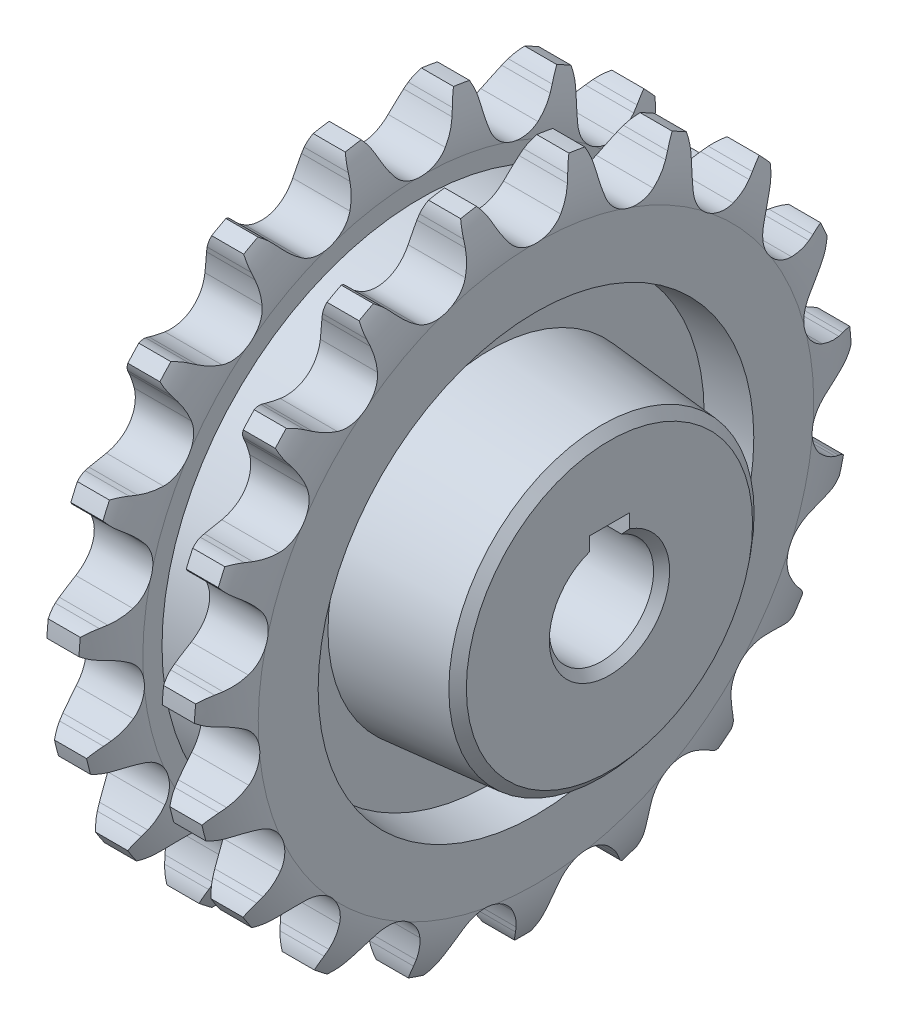
from build123d import *
from OCP.BRepFilletAPI import BRepFilletAPI_MakeChamfer

# Parameters (mm, degrees)
CUT_EXTRUDE1_DEPTH = 5.475375
CIRPATTERN1_COUNT  = 19
LPATTERN1_COUNT    = 2
LPATTERN1_PITCH    = 14.38
CHAMFER1_SIZE      = 1
CHAMFER1_SIZE2     = 1.100062868
SKETCH4_W          = 5
SKETCH4_H          = 2.799999952
CUT_EXTRUDE4_DEPTH = 71.401283385


with BuildPart() as part:
    # Sketch1 → Revolve1 (revolve)
    with BuildSketch(Plane.XY, mode=Mode.PRIVATE) as revolve1_sk:
        with BuildLine():
            Line((-3.65025, 27.149639763), (-3.65025, 34.619639763))
            ThreePointArc((-3.65025, 34.619639763), (-3.245836945, 37.918781526), (-1.99925, 41))
            Line((-1.99925, 41), (1.99925, 41))
            ThreePointArc((1.99925, 41), (3.245836945, 37.918781526), (3.65025, 34.619639763))
            Line((3.65025, 34.619639763), (3.65025, 27.149639763))
            Line((3.65025, 27.149639763), (-3.65025, 27.149639763))
        make_face()
    revolve(revolve1_sk.sketch.rotate(Axis((-6.35, 0, 0), (1, 0, 0)), 90), axis=Axis((-6.35, 0, 0), (1, 0, 0)))

    # Sketch2 → Cut-Extrude1 (cut, symmetric)
    with BuildSketch(Plane(origin=(0, 0, 0), x_dir=(0, 0, -1), z_dir=(1, 0, 0))):
        with BuildLine():
            Line((4.552244709, 38.426451297), (4.858741585, 39.1448403))
            ThreePointArc((4.858741585, 39.1448403), (5.250930322, 39.90290393), (5.750855114, 40.594675334))
            ThreePointArc((5.750855114, 40.594675334), (0, 41), (-5.750855114, 40.594675334))
            ThreePointArc((-5.750855114, 40.594675334), (-5.250930322, 39.90290393), (-4.858741585, 39.1448403))
            Line((-4.858741585, 39.1448403), (-4.552244709, 38.426451297))
            ThreePointArc((-4.552244709, 38.426451297), (-3.937302758, 37.212676935), (-3.168676608, 36.089905522))
            ThreePointArc((-3.168676608, 36.089905522), (0, 34.549839763), (3.168676608, 36.089905522))
            ThreePointArc((3.168676608, 36.089905522), (3.937302758, 37.212676935), (4.552244709, 38.426451297))
        make_face()
    cut_extrude1 = extrude(amount=CUT_EXTRUDE1_DEPTH, both=True, mode=Mode.SUBTRACT)

    # CirPattern1: Cut-Extrude1 ×19 about axis
    cirpattern1_axis = Axis((0, 0, 0), (1, 0, 0))
    for i in range(1, CIRPATTERN1_COUNT):
        add(cut_extrude1.rotate(cirpattern1_axis, i * 360 / CIRPATTERN1_COUNT), mode=Mode.SUBTRACT)


with BuildPart() as lpattern1_1:
    # LPattern1: pattern copy
    add(part.part.moved(Location(Vector(1, 0, 0) * (1 * LPATTERN1_PITCH))))


with BuildPart() as part_1:
    add(part.part)

    # Sketch5 → Revolve2 (revolve)
    with BuildSketch(Plane.XY, mode=Mode.PRIVATE) as revolve2_sk:
        Polygon((-12.81, 6.5), (27.19, 6.5), (27.19, 18.938259462), (12.34, 20.237466115), (12.34, 26.651807396), (18.03025, 27.149639763), (10.72975, 32.229639763), (3.65025, 32.229639763), (-3.65025, 27.149639763), (2.04, 26.651807396), (2.04, 20.237466115), (-12.81, 18.938259462), align=None)
    revolve(revolve2_sk.sketch.rotate(Axis((0, 0, 0), (-1, 0, 0)), 90), axis=Axis((0, 0, 0), (-1, 0, 0)))

    # Chamfer1: one chamfer whose edges measure the first distance from different faces: ONE call of the kernel's chamfer builder (chamfer() names one face for all edges)
    chamfer1_edges_1 = [part_1.edges().sort_by_distance(p)[0] for p in [
        (-12.81, 0, 6.5),
        (27.19, 0, 6.5),
    ]]
    chamfer1_edges_2 = [part_1.edges().sort_by_distance(p)[0] for p in [
        (-12.81, 0, 18.938259462),
    ]]
    chamfer1_side_2 = [part_1.faces().sort_by_distance(p)[0] for p in [
        (-12.81, 0, 18.402604594),
    ]]
    chamfer1_edges_3 = [part_1.edges().sort_by_distance(p)[0] for p in [
        (27.19, 0, 18.938259462),
    ]]
    chamfer1_side_3 = [part_1.faces().sort_by_distance(p)[0] for p in [
        (19.765, 0, 19.587862789),
    ]]
    chamfer1 = BRepFilletAPI_MakeChamfer(part_1.part.solid().wrapped)
    for e in chamfer1_edges_1:
        chamfer1.Add(CHAMFER1_SIZE, e.wrapped)
    for e in chamfer1_edges_2:
        chamfer1.Add(CHAMFER1_SIZE, CHAMFER1_SIZE2, e.wrapped, chamfer1_side_2[0].wrapped)  # the first distance lies on this face
    for e in chamfer1_edges_3:
        chamfer1.Add(CHAMFER1_SIZE, CHAMFER1_SIZE2, e.wrapped, chamfer1_side_3[0].wrapped)  # the first distance lies on this face
    add(Compound.cast(chamfer1.Shape()), mode=Mode.REPLACE)

    # Sketch4 → Cut-Extrude4 (cut, through all)
    with BuildSketch(Plane.ZY.offset(12.81)):
        with Locations((0, 7.399999976)):
            Rectangle(SKETCH4_W, SKETCH4_H)
    extrude(amount=-CUT_EXTRUDE4_DEPTH, mode=Mode.SUBTRACT)


solid = Compound([lpattern1_1.part, part_1.part])
